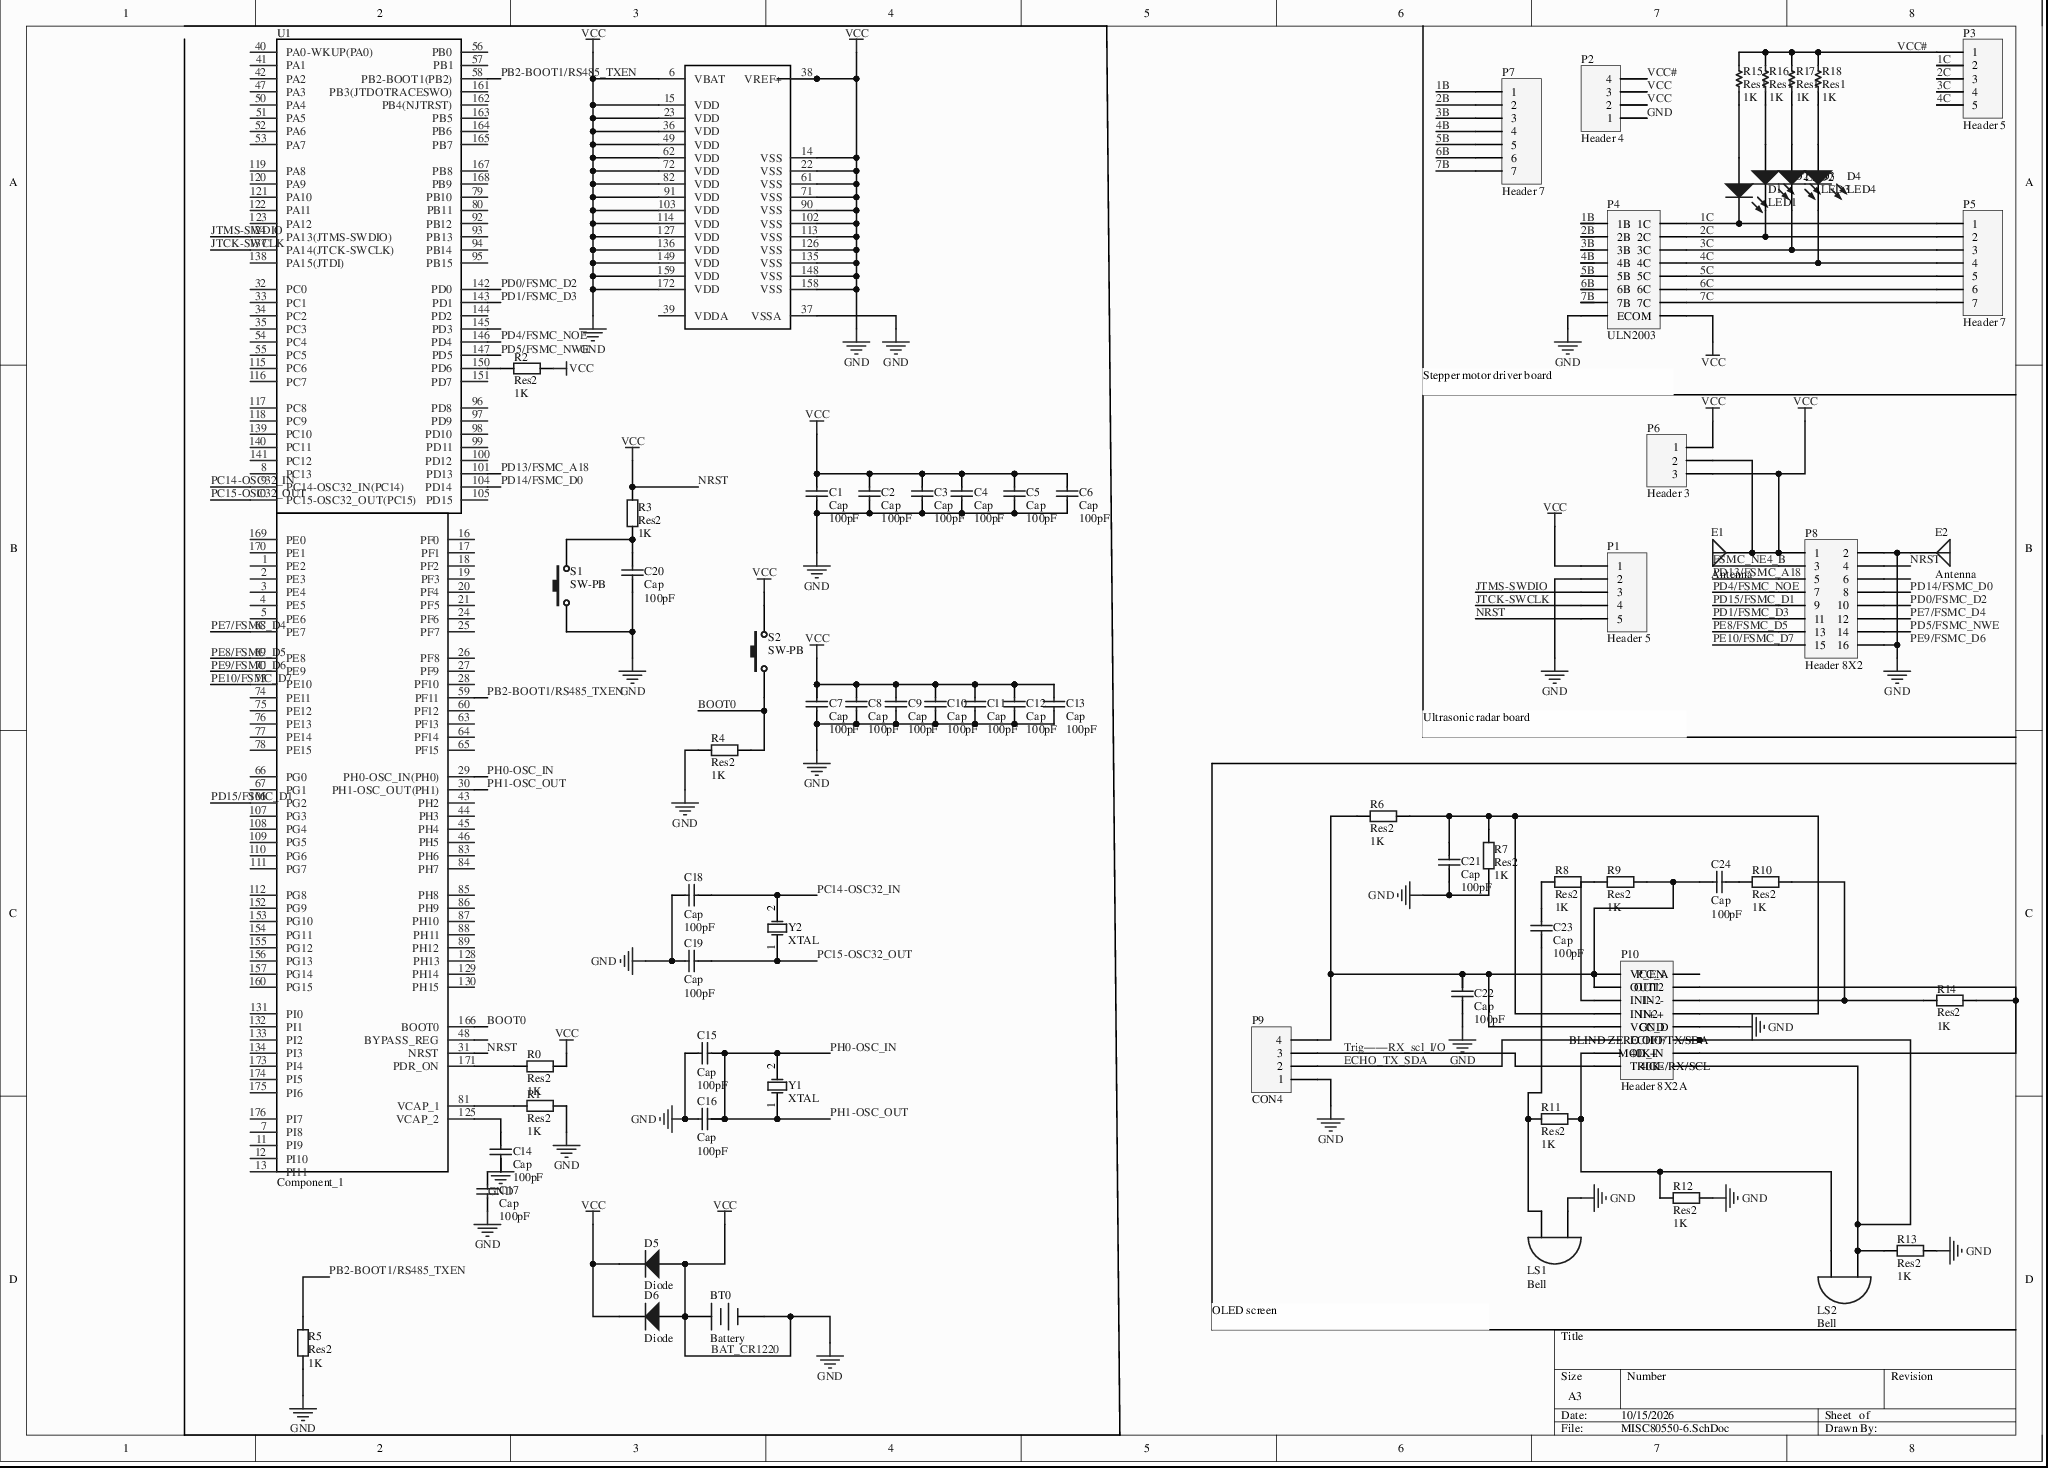
[diagram p0: MISC80550-6.SchDoc]
# Altium project MISC80550-6.PrjPcb
1 sheet, 69 parts. Net scope: global (net labels, ports and power ports of the same name join across sheets).
Board file: MISC80550.PcbDoc

## Sheet MISC80550-6.SchDoc
size A3

### Parts
BT0  Battery  [BAT-2]
C1  Cap  value 100pF  [RAD-0.3]
C2  Cap  value 100pF  [RAD-0.3]
C3  Cap  value 100pF  [RAD-0.3]
C4  Cap  value 100pF  [RAD-0.3]
C5  Cap  value 100pF  [RAD-0.3]
C6  Cap  value 100pF  [RAD-0.3]
C7  Cap  value 100pF  [RAD-0.3]
C8  Cap  value 100pF  [RAD-0.3]
C9  Cap  value 100pF  [RAD-0.3]
C10  Cap  value 100pF  [RAD-0.3]
C11  Cap  value 100pF  [RAD-0.3]
C12  Cap  value 100pF  [RAD-0.3]
C13  Cap  value 100pF  [RAD-0.3]
C14  Cap  value 100pF  [RAD-0.3]
C15  Cap  value 100pF  [RAD-0.3]
C16  Cap  value 100pF  [RAD-0.3]
C17  Cap  value 100pF  [RAD-0.3]
C18  Cap  value 100pF  [RAD-0.3]
C19  Cap  value 100pF  [RAD-0.3]
C20  Cap  value 100pF  [RAD-0.3]
C21  Cap  value 100pF  [RAD-0.3]
C22  Cap  value 100pF  [RAD-0.3]
C23  Cap  value 100pF  [RAD-0.3]
C24  Cap  value 100pF  [RAD-0.3]
D1  LED1  [LED-0]
D2  LED2  [LED-0]
D3  LED3  [LED-0]
D4  LED4  [LED-0]
D5  Diode  [DSO-C2/X3.3]
D6  Diode  [DSO-C2/X3.3]
E1  Antenna  [PIN1]
E2  Antenna  [PIN1]
LS1  Bell  [PIN2]
LS2  Bell  [PIN2]
P1  Header 5  [HDR1X5]
P2  Header 4  [HDR1X4]
P3  Header 5  [HDR1X5]
P4  ULN2003  [HDR2X8_CEN]
P5  Header 7  [HDR1X7]
P6  Header 3  [HDR1X3]
P7  Header 7  [HDR1X7]
P8  Header 8X2  [HDR2X8]
P9  CON4  [HDR1X4]
P10  Header 8X2A  [HDR2X8_CEN]
R0  Res2  value 1K  [AXIAL-0.4]
R1  Res2  value 1K  [AXIAL-0.4]
R2  Res2  value 1K  [AXIAL-0.4]
R3  Res2  value 1K  [AXIAL-0.4]
R4  Res2  value 1K  [AXIAL-0.4]
R5  Res2  value 1K  [AXIAL-0.4]
R6  Res2  value 1K  [AXIAL-0.4]
R7  Res2  value 1K  [AXIAL-0.4]
R8  Res2  value 1K  [AXIAL-0.4]
R9  Res2  value 1K  [AXIAL-0.4]
R10  Res2  value 1K  [AXIAL-0.4]
R11  Res2  value 1K  [AXIAL-0.4]
R12  Res2  value 1K  [AXIAL-0.4]
R13  Res2  value 1K  [AXIAL-0.4]
R14  Res2  value 1K  [AXIAL-0.4]
R15  Res1  value 1K  [AXIAL-0.3]
R16  Res1  value 1K  [AXIAL-0.3]
R17  Res1  value 1K  [AXIAL-0.3]
R18  Res1  value 1K  [AXIAL-0.3]
S1  SW-PB  [SPST-2]
S2  SW-PB  [SPST-2]
U1  Component_1  [PCBComponent_1]
Y1  XTAL  [BCY-W2/D3.1]
Y2  XTAL  [BCY-W2/D3.1]

### Nets
BAT_CR1220: BT0.1(+) BT0.2(-) C1.1 C1.2 C2.1 C2.2 C3.1 C3.2 C4.1 C4.2 C5.1 C5.2 C6.1 C6.2 C7.1 C7.2 C8.1 C8.2 C9.1 C9.2 C10.1 C10.2 C11.1 C11.2 C12.1 C12.2 C13.1 C13.2 C14.1 C15.1 C16.1 C17.1 C18.1 C19.1 C20.1 C21.1 C22.1 D5.1(A) D5.2(K) D6.1(A) D6.2(K) E1.1(A) E2.1(A) LS1.1(A) P1.1 P1.2 P1.5 P2.1 P2.2 P2.3 P4.8(E) P4.16(COM) P6.1(3) P6.2 P6.3(1) P8.1 P8.2 P8.4 P8.16 P9.1 P10.13(GND) R0.2 R1.2 R2.2 R3.2 R4.1 R5.1 R7.1 R12.1 R13.1 S1.1 S2.2 U1.6(VBAT) U1.14(VSS) U1.15(VDD) U1.22(VSS) U1.23(VDD) U1.31(NRST) U1.36(VDD) U1.37(VSSA) U1.38(VREF+) U1.49(VDD) U1.61(VSS) U1.62(VDD) U1.71(VSS) U1.72(VDD) U1.82(VDD) U1.90(VSS) U1.91(VDD) U1.102(VSS) U1.103(VDD) U1.113(VSS) U1.114(VDD) U1.126(VSS) U1.127(VDD) U1.135(VSS) U1.136(VDD) U1.148(VSS) U1.149(VDD) U1.158(VSS) U1.159(VDD) U1.172(VDD)  [also labelled GND, NRST, VCC]
1B: P4.1(1B) P7.1
1C: D1.2(K) P3.2 P4.9(1C) P5.1
2B: P4.2(2B) P7.2
2C: D2.2(K) P3.3 P4.10(2C) P5.2
3B: P4.3(3B) P7.3
3C: D3.2(K) P3.4 P4.11(3C) P5.3
4B: P4.4(4B) P7.4
4C: D4.2(K) P3.5 P4.12(4C) P5.4
5B: P4.5(5B) P7.5
5C: P4.13(5C) P5.5
6B: P4.6(6B) P7.6
6C: P4.14(6C) P5.6
7B: P4.7(7B) P7.7
7C: P4.15(7C) P5.7
BOOT0: R4.2 S2.1 U1.166(BOOT0)
ECHO_TX_SDA: P9.2 P10.6(ECHO/TX/SDA)
FSMC_NE4_B: P8.3
JTCK-SWCLK: P1.4 U1.137(PA14(JTCK-SWCLK))
JTMS-SWDIO: P1.3 U1.124(PA13(JTMS-SWDIO))
PB2-BOOT1/RS485_TXEN: R5.2 U1.58(PB2-BOOT1(PB2)) U1.59(PF11)
PC14-OSC32_IN: C18.2 U1.9(PC14-OSC32_IN(PC14)) Y2.2(OSC2)
PC15-OSC32_OUT: C19.2 U1.10(PC15-OSC32_OUT(PC15)) Y2.1(OSC1)
PD0/FSMC_D2: P8.10 U1.142(PD0)
PD1/FSMC_D3: P8.11 U1.143(PD1)
PD4/FSMC_NOE: P8.7 U1.146(PD4)
PD5/FSMC_NWE: P8.14 U1.147(PD5)
PD13/FSMC_A18: P8.5 U1.101(PD13)
PD14/FSMC_D0: P8.8 U1.104(PD14)
PD15/FSMC_D1: P8.9 U1.106(PG2)
PE7/FSMC_D4: P8.12 U1.68(PE7)
PE8/FSMC_D5: P8.13 U1.69(PE8)
PE9/FSMC_D6: U1.70(PE9)
PE10/FSMC_D7: P8.15 U1.73(PE10)
PH0-OSC_IN: C15.2 C16.2 U1.29(PH0-OSC_IN(PH0)) U1.30(PH1-OSC_OUT(PH1)) Y1.1(OSC1) Y1.2(OSC2)  [also labelled PH1-OSC_OUT]
Trig——RX_scl_I/O: P9.3 P10.8(TRIGE/RX/SCL)
VCC#: P2.4 P3.1 R15.2 R16.2 R17.2 R18.2
NetC14_2: C14.2 U1.125(VCAP_2)
NetC20_2: C20.2 R3.1 S1.2
NetC21_2: C21.2 P10.4(IN1+) P10.12(IN2+) R6.2 R7.2
NetC22_2: C22.2 C24.2 P9.4 P10.1(VCC_A) P10.2(OUT1) P10.5(VCC_D) R6.1 R9.1
NetC23_1: C23.1 LS1.2(B) R11.2
NetC23_2: C23.2 R8.2
NetC24_1: C24.1 R10.2
NetD1_1: D1.1(A) R15.1
NetD2_1: D2.1(A) R16.1
NetD3_1: D3.1(A) R17.1
NetD4_1: D4.1(A) R18.1
NetLS2_1: LS2.1(A) P10.14(BLIND_ZERO_OFF) P10.16(40K-) R13.2
NetLS2_2: LS2.2(B) P10.7(40K+) R11.1 R12.2
NetP10_10: P10.10(OUT2) P10.15(MOD_IN) R14.1
NetP10_11: P10.11(IN2-) R10.1 R14.2
NetR0_1: R0.1 U1.171(PDR_ON)
NetR1_1: R1.1 U1.81(VCAP_1)
NetR2_1: R2.1 U1.150(PD6)
NetR8_1: R8.1 R9.2

Not connected (* = marked no-connect by the designer): C17 2; P8 6; P10 3(IN1-) 9(P_EN); U1 1(PE2) 2(PE3) 3(PE4) 4(PE5) 5(PE6) 7(PI8) 8(PC13) 11(PI9) 12(PI10) 13(PI11) 16(PF0) 17(PF1) 18(PF2) 19(PF3) 20(PF4) 21(PF5) 24(PF6) 25(PF7) 26(PF8) 27(PF9) 28(PF10) 32(PC0) 33(PC1) 34(PC2) 35(PC3) 39(VDDA) 40(PA0-WKUP(PA0)) 41(PA1) 42(PA2) 43(PH2) 44(PH3) 45(PH4) 46(PH5) 47(PA3) 48(BYPASS_REG) 50(PA4) 51(PA5) 52(PA6) 53(PA7) 54(PC4) 55(PC5) 56(PB0) 57(PB1) 60(PF12) 63(PF13) 64(PF14) 65(PF15) 66(PG0) 67(PG1) 74(PE11) 75(PE12) 76(PE13) 77(PE14) 78(PE15) 79(PB10) 80(PB11) 83(PH6) 84(PH7) 85(PH8) 86(PH9) 87(PH10) 88(PH11) 89(PH12) 92(PB12) 93(PB13) 94(PB14) 95(PB15) 96(PD8) 97(PD9) 98(PD10) 99(PD11) 100(PD12) 105(PD15) 107(PG3) 108(PG4) 109(PG5) 110(PG6) 111(PG7) 112(PG8) 115(PC6) 116(PC7) 117(PC8) 118(PC9) 119(PA8) 120(PA9) 121(PA10) 122(PA11) 123(PA12) 128(PH13) 129(PH14) 130(PH15) 131(PI0) 132(PI1) 133(PI2) 134(PI3) 138(PA15(JTDI)) 139(PC10) 140(PC11) 141(PC12) 144(PD2) 145(PD3) 151(PD7) 152(PG9) 153(PG10) 154(PG11) 155(PG12) 156(PG13) 157(PG14) 160(PG15) 161(PB3(JTDOTRACESWO)) 162(PB4(NJTRST)) 163(PB5) 164(PB6) 165(PB7) 167(PB8) 168(PB9) 169(PE0) 170(PE1) 173(PI4) 174(PI5) 175(PI6) 176(PI7)

### Notes on the sheet
- Stepper motor driver board
- Ultrasonic radar board
- OLED screen
- Labels drawn without touching a wire or pin: PE9/FSMC_D6

### Library data of the parts
BT0 = Battery: Multicell Battery; Published: 24-Mar-1999; LatestRevisionDate: 17-Jul-2002; LatestRevisionNote: Re-released for DXP Platform.; PackageReference: BAT-2; Publisher: Altium Limited
C1-C24 = Cap: Capacitor; Published: 8-Jun-2000; LatestRevisionDate: 17-Jul-2002; LatestRevisionNote: Re-released for DXP Platform.; PackageReference: RAD-0.3; Publisher: Altium Limited
D1-D4 = LED0: Typical INFRARED GaAs LED; Published: 8-Jun-2000; LatestRevisionDate: 08-Jul-2005; LatestRevisionNote: Mech Layer 1 removed.; PackageReference: LED-0; Publisher: Altium Limited
D5 D6 = Diode: Default Diode; Published: 8-Jun-2000; LatestRevisionDate: 17-Jul-2002; LatestRevisionNote: Re-released for DXP Platform.; PackageVersion: Sep-1996; PackageReference: SMC; Code_JEDEC: DO-214-AB; Publisher: Altium Limited
E1 E2 = Antenna: Generic Antenna; Published: 24-Mar-1999; LatestRevisionDate: 17-Jul-2002; LatestRevisionNote: Re-released for DXP Platform.; PackageReference: PIN1; Publisher: Altium Limited
LS1 LS2 = Bell: Electrical Bell; Published: 24-Mar-1999; LatestRevisionDate: 17-Jul-2002; LatestRevisionNote: Re-released for DXP Platform.; PackageReference: PIN2; Publisher: Altium Limited
P1 P3 = Header 5: Header, 5-Pin; LatestRevisionDate: 17-Jul-2002; LatestRevisionNote: Re-released for DXP Platform.; Publisher: Altium Limited
P2 P9 = Header 4: Header, 4-Pin; LatestRevisionDate: 17-Jul-2002; LatestRevisionNote: Re-released for DXP Platform.; Publisher: Altium Limited
P4 = Header 8X2A: ULN2003, Dual row; LatestRevisionDate: 17-Jul-2002; LatestRevisionNote: Re-released for DXP Platform.; Publisher: Altium Limited
P5 P7 = Header 7: Header, 7-Pin; LatestRevisionDate: 17-Jul-2002; LatestRevisionNote: Re-released for DXP Platform.; Publisher: Altium Limited
P6 = Header 3: Header, 3-Pin; LatestRevisionDate: 17-Jul-2002; LatestRevisionNote: Re-released for DXP Platform.; Publisher: Altium Limited
P8 = Header 8X2: Header, 8-Pin, Dual row; LatestRevisionDate: 17-Jul-2002; LatestRevisionNote: Re-released for DXP Platform.; Publisher: Altium Limited
P10 = Header 8X2A: Header, 8-Pin, Dual row; LatestRevisionDate: 17-Jul-2002; LatestRevisionNote: Re-released for DXP Platform.; Publisher: Altium Limited
R0-R14 = Res2: Resistor; Published: 8-Jun-2000; LatestRevisionDate: 17-Jul-2002; LatestRevisionNote: Re-released for DXP Platform.; PackageReference: AXIAL-0.4; Publisher: Altium Limited
R15-R18 = Res1: Resistor; Published: 8-Jun-2000; LatestRevisionDate: 17-Jul-2002; LatestRevisionNote: Re-released for DXP Platform.; PackageReference: AXIAL-0.3; Publisher: Altium Limited
S1 S2 = SW-PB: Switch; Published: 24-Mar-1999; LatestRevisionDate: 17-Jul-2002; LatestRevisionNote: Re-released for DXP Platform.; PackageReference: SPST-2; Publisher: Altium Limited
Y1 Y2 = XTAL: Crystal Oscillator; Published: 8-Jun-2000; LatestRevisionDate: 17-Jul-2002; LatestRevisionNote: Re-released for DXP Platform.; PackageReference: R38; Publisher: Altium Limited